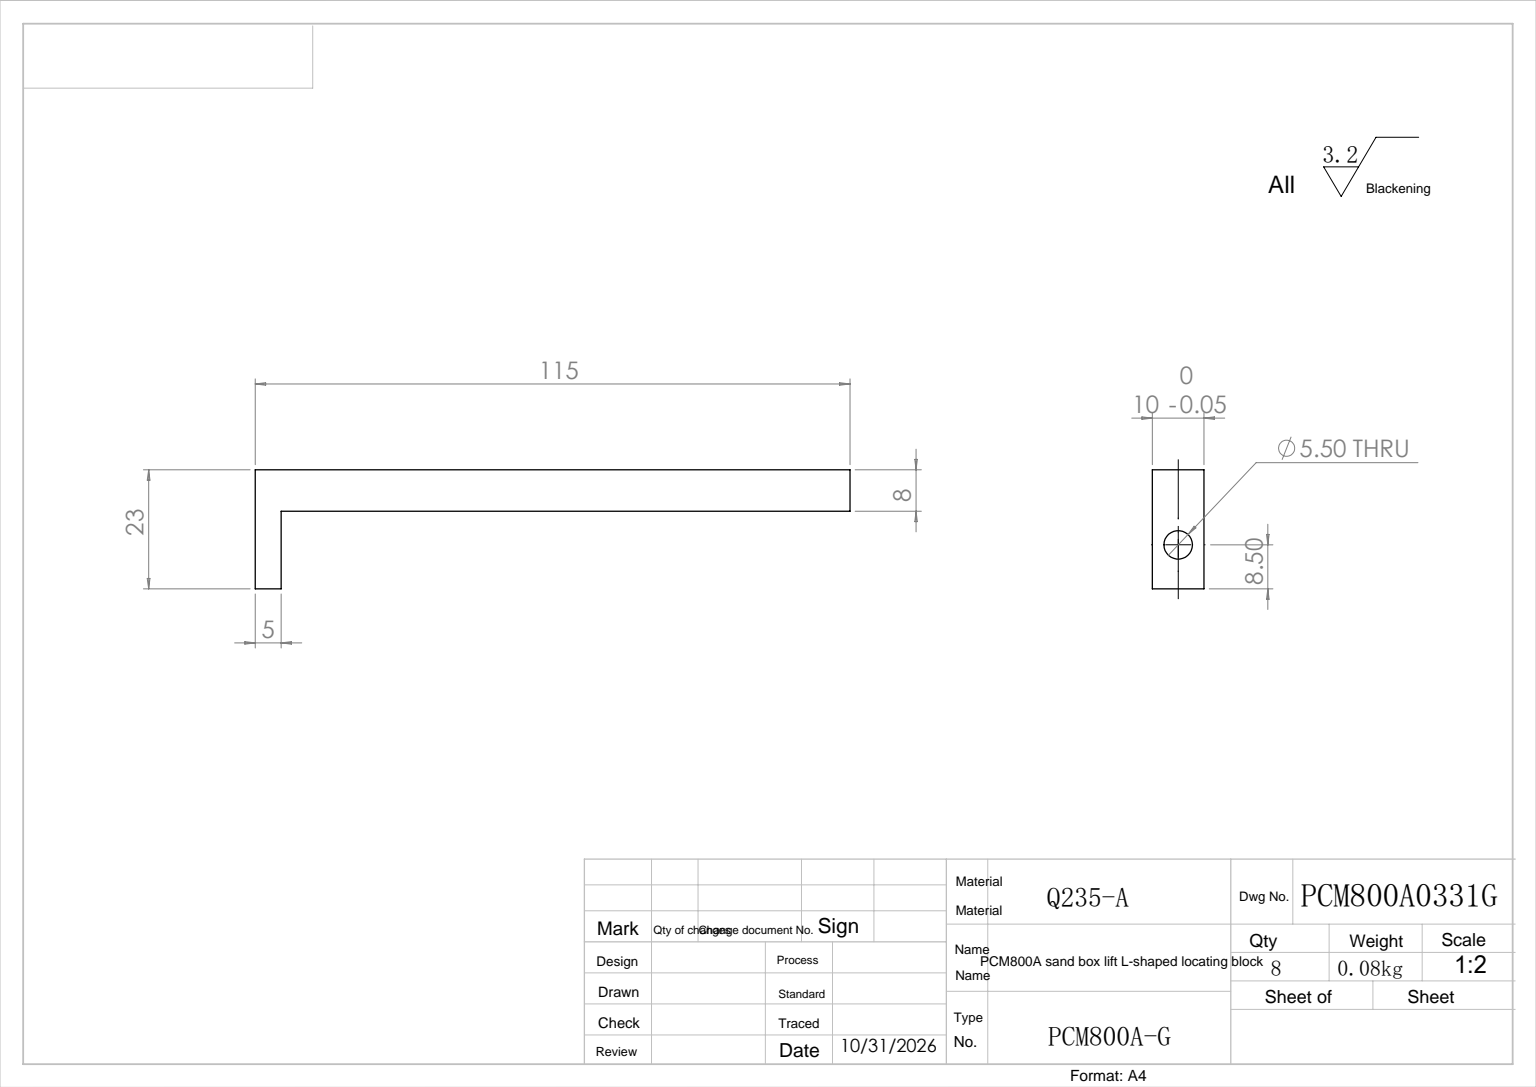
from build123d import *

# Parameters (mm, degrees)
EXTRUDE_1_DEPTH     = 10
SKETCH_2_R          = 2.75
CUT_EXTRUDE_1_DEPTH = 117.404467268


with BuildPart() as part:
    # 草图1 → 凸台-拉伸1 (new body)
    with BuildSketch(Plane.XY):
        Polygon((0, 0), (0, -110), (15, -110), (15, -115), (-8, -115), (-8, 0), align=None)
    extrude(amount=EXTRUDE_1_DEPTH)

    # 草图2 → 切除-拉伸1 (cut, through all)
    with BuildSketch(Plane.XZ.offset(115)):
        with Locations(Location((6.5, 5, 0), (0, 0, 270))):
            Circle(SKETCH_2_R)
    extrude(amount=-CUT_EXTRUDE_1_DEPTH, mode=Mode.SUBTRACT)


solid = part.part
